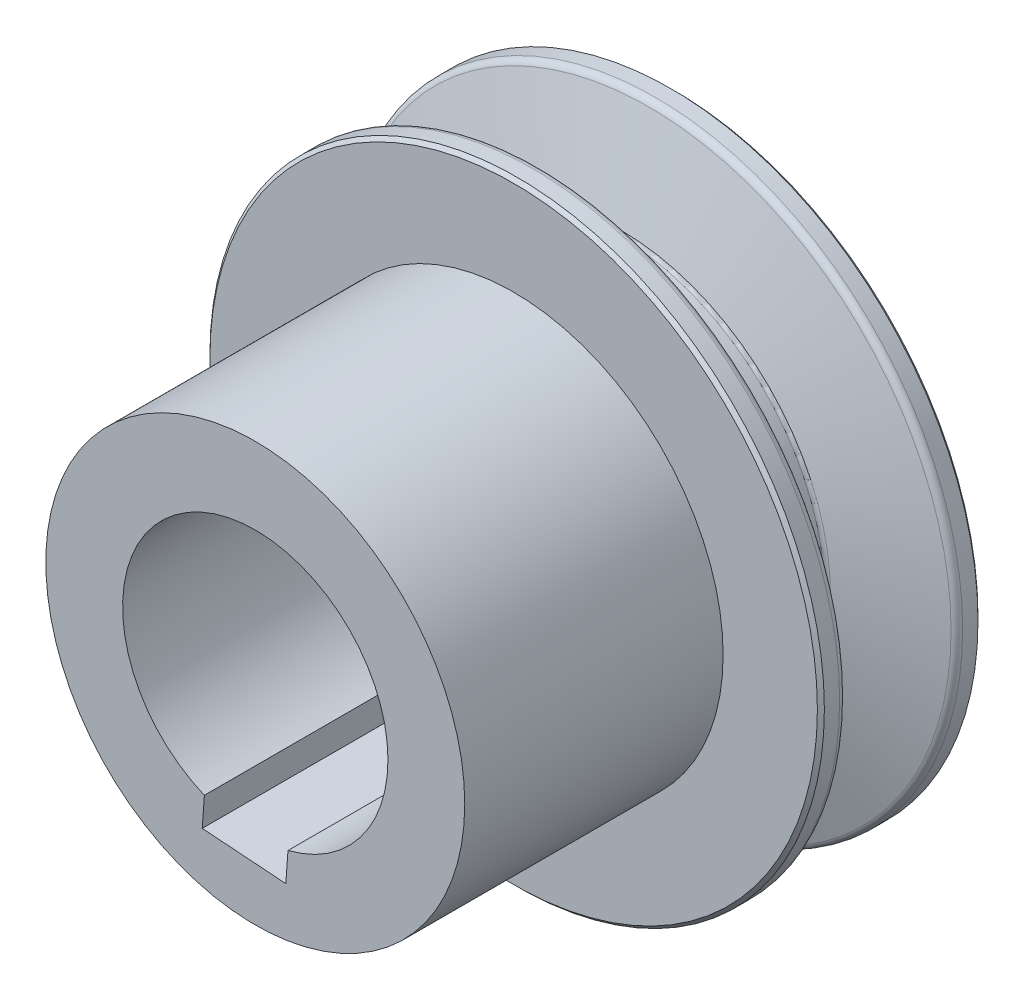
from build123d import *

# Parameters (mm, degrees)
SKETCH2_R           = 30
BOSS_EXTRUDE1_DEPTH = 37
CUT_EXTRUDE1_DEPTH  = 627.690359496
SKETCH4_W           = 19
SKETCH4_H           = 60
CHAMFER1_SIZE       = 0.5
FILLET1_R           = 0.5
FILLET2_R           = 1


with BuildPart() as part:
    # Sketch1 → Revolve1 (revolve)
    with BuildSketch(Plane(origin=(0, 22.743963655, 0), x_dir=(1, 0, 0), z_dir=(0, 1, 0))):
        Polygon((620.230642584, 121.692981355), (576.230642584, 121.692981355), (576.230642584, 98.692981355), (620.230642584, 98.692981355), (620.230642584, 102.12292397), (605.930642584, 106.494872715), (605.930642584, 113.891089995), (620.230642584, 118.26303874), align=None)
    revolve(axis=Axis((576.230642584, 22.743963655, -121.692981355), (0, 0, 1)))

    # Sketch2 → Boss-Extrude1 (add)
    with BuildSketch(Plane.XY.offset(-98.692981355)):
        with Locations((576.230642584, 22.743963655)):
            Circle(SKETCH2_R)
    extrude(amount=BOSS_EXTRUDE1_DEPTH)

    # Sketch3 → Cut-Extrude1 (cut, through all)
    with BuildSketch(Plane(origin=(0, 0, -121.692981355), x_dir=(-1, 0, 0), z_dir=(0, 0, -1))):
        with BuildLine():
            Line((-580.602866602, 0.068566036), (-568.634263156, 0.936051797))
            Line((-568.634263156, 0.936051797), (-568.943105698, 5.197117609))
            ThreePointArc((-568.943105698, 5.197117609), (-574.857123463, 3.793674865), (-580.911709145, 4.329631849))
            Line((-580.911709145, 4.329631849), (-580.602866602, 0.068566036))
        make_face()
    extrude(amount=-CUT_EXTRUDE1_DEPTH, mode=Mode.SUBTRACT)

    # Sketch4 → Cut-Revolve1 (revolve, cut)
    with BuildSketch(Plane.XZ.offset(-22.743963655)):
        with Locations((585.730642584, -91.692981355)):
            Rectangle(SKETCH4_W, SKETCH4_H)
    revolve(axis=Axis((576.230642584, 22.743963655, -61.692981355), (0, 0, -1)), mode=Mode.SUBTRACT)

    # Chamfer1
    chamfer1_edges = [part.edges().sort_by_distance(p)[0] for p in [
        (532.230642584, 22.743963655, -98.692981355),
        (532.230642584, 22.743963655, -121.692981355),
    ]]
    chamfer(chamfer1_edges, length=CHAMFER1_SIZE)

    # Fillet1
    fillet1_edges = [part.edges().sort_by_distance(p)[0] for p in [
        (546.530642584, 22.743963655, -113.891089995),
        (546.530642584, 22.743963655, -106.494872715),
    ]]
    fillet(fillet1_edges, radius=FILLET1_R)

    # Fillet2
    fillet2_edges = [part.edges().sort_by_distance(p)[0] for p in [
        (532.230642584, 22.743963655, -118.26303874),
        (532.230642584, 22.743963655, -102.12292397),
    ]]
    fillet(fillet2_edges, radius=FILLET2_R)


solid = part.part
